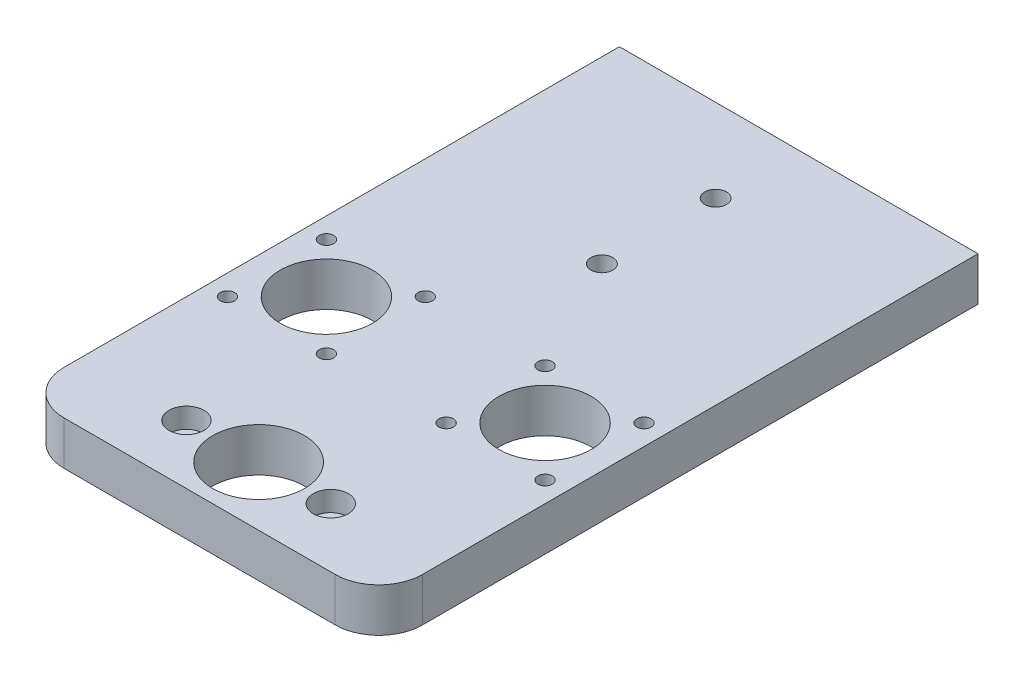
from build123d import *

# Parameters (mm, degrees)
SKETCH_1_W                = 82
SKETCH_1_H                = 137
EXTRUDE_1_DEPTH           = 10
SKETCH_4_R                = 10.5
CUT_EXTRUDE_3_DEPTH       = 81.456509991
FILLET_9_R                = 10
HOLE_WIZARD_2_D           = 4.3
HOLE_WIZARD_2_CBORE_D     = 8
HOLE_WIZARD_2_CBORE_DEPTH = 4.6
HOLE_WIZARD_M4_2_D        = 3.3
HOLE_WIZARD_M4_2_DEPTH    = 18.5
HOLE_WIZARD_M4_2_TIP      = 0.991420021
MM_2_D                    = 21.1
HOLE_WIZARD_M4_3_D        = 3.3
MM_2_2_D                  = 5
MM_2_2_DEPTH              = 10.1
MM_2_2_TIP                = 1.502151548
HOLE_WIZARD_M6_1_D        = 5
HOLE_WIZARD_M6_1_DEPTH    = 15
HOLE_WIZARD_M6_1_TIP      = 1.502151548
HOLE_WIZARD_M6_4_D        = 5


with BuildPart() as part:
    # 草图1 → 凸台-拉伸1 (new body)
    with BuildSketch(Plane(origin=(0, 0, 0), x_dir=(1, 0, 0), z_dir=(0, 1, 0))):
        Rectangle(SKETCH_1_W, SKETCH_1_H)
    extrude(amount=EXTRUDE_1_DEPTH)

    # 草图4 → 切除-拉伸3 (cut, through all)
    with BuildSketch(Plane(origin=(0, 10, 0), x_dir=(1, 0, 0), z_dir=(0, 1, 0))):
        with Locations(Location((0, -55, 0), (0, 0, 270))):
            Circle(SKETCH_4_R)
    extrude(amount=-CUT_EXTRUDE_3_DEPTH, mode=Mode.SUBTRACT)

    # 圆角9
    fillet_9_edges = [part.edges().sort_by_distance(p)[0] for p in [
        (41, 5, 68.5),
        (-41, 5, 68.5),
    ]]
    fillet(fillet_9_edges, radius=FILLET_9_R)

    # 打孔尺寸(%根据)开槽圆柱头螺钉的类型2 (through all)
    with Locations(Plane(origin=(0, 10, 0), x_dir=(1, 0, 0), z_dir=(0, 1, 0))):
        with Locations((-16.5, -55), (16.5, -55)):
            CounterBoreHole(HOLE_WIZARD_2_D / 2, HOLE_WIZARD_2_CBORE_D / 2, HOLE_WIZARD_2_CBORE_DEPTH)

    # M4 螺纹孔2
    with Locations(Plane(origin=(0, 0, -68.5), x_dir=(-1, 0, 0), z_dir=(0, 0, -1))):
        with Locations((-15, 5), (15, 5)):
            Hole(HOLE_WIZARD_M4_2_D / 2, depth=HOLE_WIZARD_M4_2_DEPTH)
            with Locations((0, 0, -(HOLE_WIZARD_M4_2_DEPTH + HOLE_WIZARD_M4_2_TIP / 2))):  # 118° drill point
                Cone(0, HOLE_WIZARD_M4_2_D / 2, HOLE_WIZARD_M4_2_TIP, mode=Mode.SUBTRACT)

    # mm _2 (through all)
    with Locations(Plane(origin=(0, 10, 0), x_dir=(1, 0, 0), z_dir=(0, 1, 0))):
        with Locations((-25, -14.5), (25, -14.5)):
            Hole(MM_2_D / 2)

    # M4 螺纹孔3 (through all)
    with Locations(Plane(origin=(0, 0, 0), x_dir=(-1, 0, 0), z_dir=(0, -1, 0))):
        with Locations((-13.686291501, -3.186291501), (-36.313708499, -3.186291501), (-36.313708499, -25.813708499), (-13.686291501, -25.813708499)):
            hole_wizard_m4_3 = Hole(HOLE_WIZARD_M4_3_D / 2)

    # 镜向2: M4 螺纹孔3 across plane
    add(hole_wizard_m4_3.mirror(Plane(origin=(0, 0, 0), x_dir=(0, 0, 1), z_dir=(1, 0, 0))), mode=Mode.SUBTRACT)

    # mm _2 2
    with Locations(Plane(origin=(0, 0, -68.5), x_dir=(-1, 0, 0), z_dir=(0, 0, -1))):
        with Locations((32.5, 5), (-32.5, 5)):
            Hole(MM_2_2_D / 2, depth=MM_2_2_DEPTH)
            with Locations((0, 0, -(MM_2_2_DEPTH + MM_2_2_TIP / 2))):  # 118° drill point
                Cone(0, MM_2_2_D / 2, MM_2_2_TIP, mode=Mode.SUBTRACT)

    # M6 螺纹孔1
    with Locations(Plane(origin=(0, 10, 0), x_dir=(1, 0, 0), z_dir=(0, 1, 0))):
        with Locations((0, 49.5)):
            Hole(HOLE_WIZARD_M6_1_D / 2, depth=HOLE_WIZARD_M6_1_DEPTH)
            with Locations((0, 0, -(HOLE_WIZARD_M6_1_DEPTH + HOLE_WIZARD_M6_1_TIP / 2))):  # 118° drill point
                Cone(0, HOLE_WIZARD_M6_1_D / 2, HOLE_WIZARD_M6_1_TIP, mode=Mode.SUBTRACT)

    # M6 螺纹孔4 (through all)
    with Locations(Plane(origin=(0, 10, 0), x_dir=(1, 0, 0), z_dir=(0, 1, 0))):
        with Locations((0, 23.5)):
            Hole(HOLE_WIZARD_M6_4_D / 2)


solid = part.part
